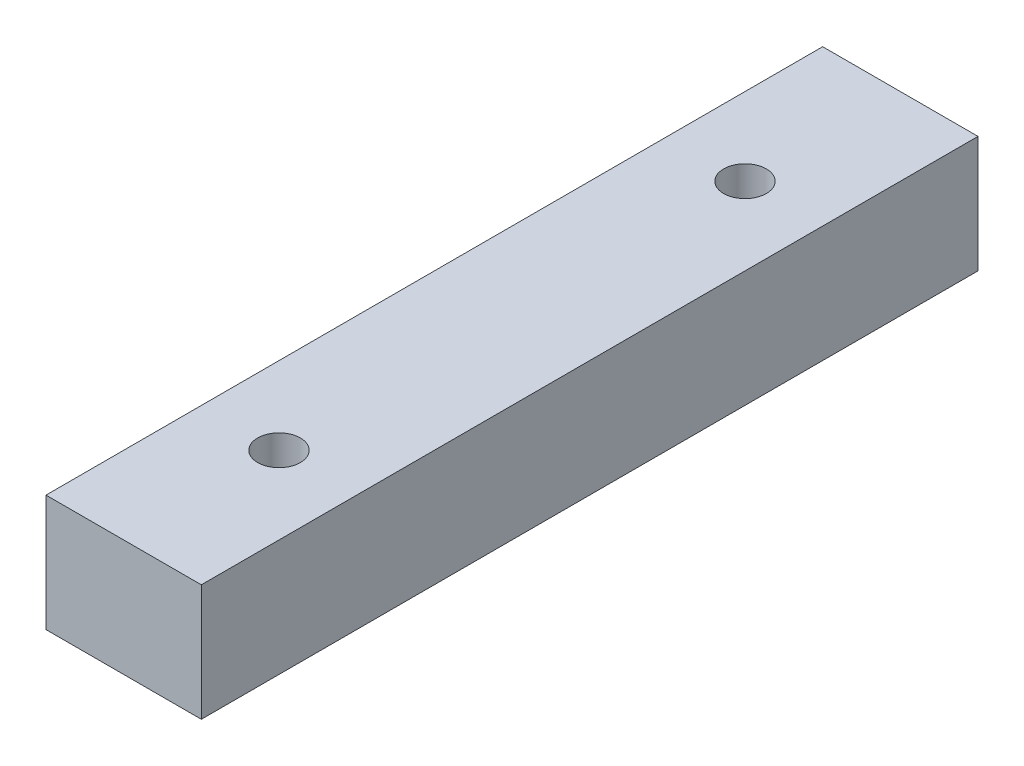
from build123d import *

# Parameters (mm, degrees)
SKETCH_1_W                = 40
SKETCH_1_H                = 200
EXTRUDE_1_DEPTH           = 15
HOLE_WIZARD_1_D           = 6.6
HOLE_WIZARD_1_CBORE_D     = 11
HOLE_WIZARD_1_CBORE_DEPTH = 10


with BuildPart() as part:
    # 草图1 → 凸台-拉伸1 (new, symmetric)
    with BuildSketch(Plane(origin=(0, 0, 0), x_dir=(1, 0, 0), z_dir=(0, 1, 0))):
        Rectangle(SKETCH_1_W, SKETCH_1_H)
    extrude(amount=EXTRUDE_1_DEPTH, both=True)

    # 打孔尺寸(%根据)内六角圆柱头螺钉的类型1 (through all)
    with Locations(Plane(origin=(0, 15, 0), x_dir=(1, 0, 0), z_dir=(0, 1, 0))):
        with Locations((0, 60), (0, -60)):
            CounterBoreHole(HOLE_WIZARD_1_D / 2, HOLE_WIZARD_1_CBORE_D / 2, HOLE_WIZARD_1_CBORE_DEPTH)


solid = part.part
